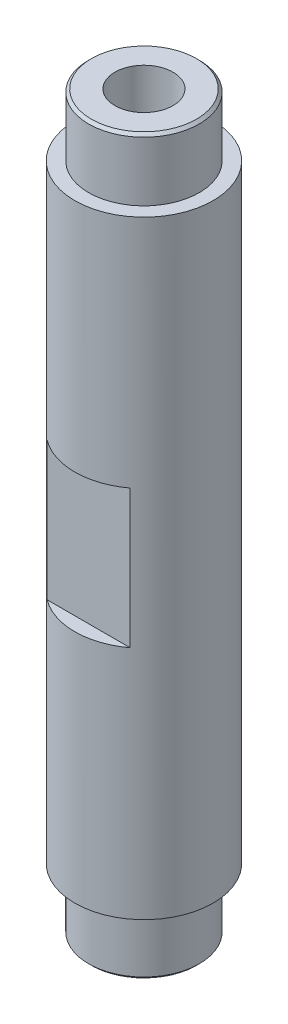
from build123d import *

# Parameters (mm, degrees)
SKETCH1_W           = 5
SKETCH1_H           = 53
SKETCH4_OUTSIDE_W   = 22.97
SKETCH4_OUTSIDE_H   = 22.97
SKETCH4_OUTSIDE_R   = 4
EXTRUDE1_DEPTH      = 4.5
SKETCH5_OUTSIDE_W   = 22.97
SKETCH5_OUTSIDE_H   = 22.97
SKETCH5_OUTSIDE_R   = 4
EXTRUDE2_DEPTH      = 4.5
EXTRUDE3_DEPTH      = 28.427176304
EXTRUDE3_DEPTH_BACK = 28.427176304
SKETCH6_W           = 7.231066263
SKETCH6_H           = 10
SKETCH6_W_2         = 2.606547141
CHAMFER1_SIZE       = 0.2


with BuildPart() as part:
    # Sketch1 → Revolve1 (revolve)
    with BuildSketch(Plane(origin=(0, 0, 0), x_dir=(0, 0, -1), z_dir=(1, 0, 0))):
        with Locations((-2.5, 0)):
            Rectangle(SKETCH1_W, SKETCH1_H)
    revolve(axis=Axis((0, 26.5, 0), (0, -1, 0)))

    # Sketch2 → M5 Tapped Hole1 (revolve, cut)
    with BuildSketch(Plane(origin=(0, 26.5, 0), x_dir=(0, 0, 1), z_dir=(1, 0, 0))):
        Polygon((0, 0), (0, 11.6618073), (2.1, 10.4), (2.1, 0), align=None)
    m5_tapped_hole1 = revolve(axis=Axis((0, 32.85, 0), (0, -1, 0)), mode=Mode.SUBTRACT)

    # Mirror1: M5 Tapped Hole1 across plane
    add(m5_tapped_hole1.mirror(Plane.ZX), mode=Mode.SUBTRACT)

    # Sketch4 outside → Extrude1 (cut)
    with BuildSketch(Plane.XZ.offset(26.5)):
        Rectangle(SKETCH4_OUTSIDE_W, SKETCH4_OUTSIDE_H)
        with Locations(Location((0, 0, 0), (0, 0, 270))):
            Circle(SKETCH4_OUTSIDE_R, mode=Mode.SUBTRACT)
    extrude(amount=-EXTRUDE1_DEPTH, mode=Mode.SUBTRACT)

    # Sketch5 outside → Extrude2 (cut)
    with BuildSketch(Plane(origin=(0, 26.5, 0), x_dir=(1, 0, 0), z_dir=(0, 1, 0))):
        Rectangle(SKETCH5_OUTSIDE_W, SKETCH5_OUTSIDE_H)
        with Locations(Location((0, 0, 0), (0, 0, 90))):
            Circle(SKETCH5_OUTSIDE_R, mode=Mode.SUBTRACT)
    extrude(amount=-EXTRUDE2_DEPTH, mode=Mode.SUBTRACT)

    # Sketch6 → Extrude3 (cut, two sides: drawn at the far end of the back side and taken through both)
    with BuildSketch(Plane(origin=(0, 0, 0), x_dir=(0, 0, -1), z_dir=(1, 0, 0)).offset(-EXTRUDE3_DEPTH_BACK)):
        with Locations((-7.615533132, 0)):
            Rectangle(SKETCH6_W, SKETCH6_H)
        with Locations((5.303273571, 0)):
            Rectangle(SKETCH6_W_2, SKETCH6_H)
    extrude(amount=EXTRUDE3_DEPTH + EXTRUDE3_DEPTH_BACK, mode=Mode.SUBTRACT)

    # Chamfer1
    chamfer1_edges = [part.edges().sort_by_distance(p)[0] for p in [
        (0, -26.5, 4),
        (0, 26.5, 4),
    ]]
    chamfer(chamfer1_edges, length=CHAMFER1_SIZE)


solid = part.part
